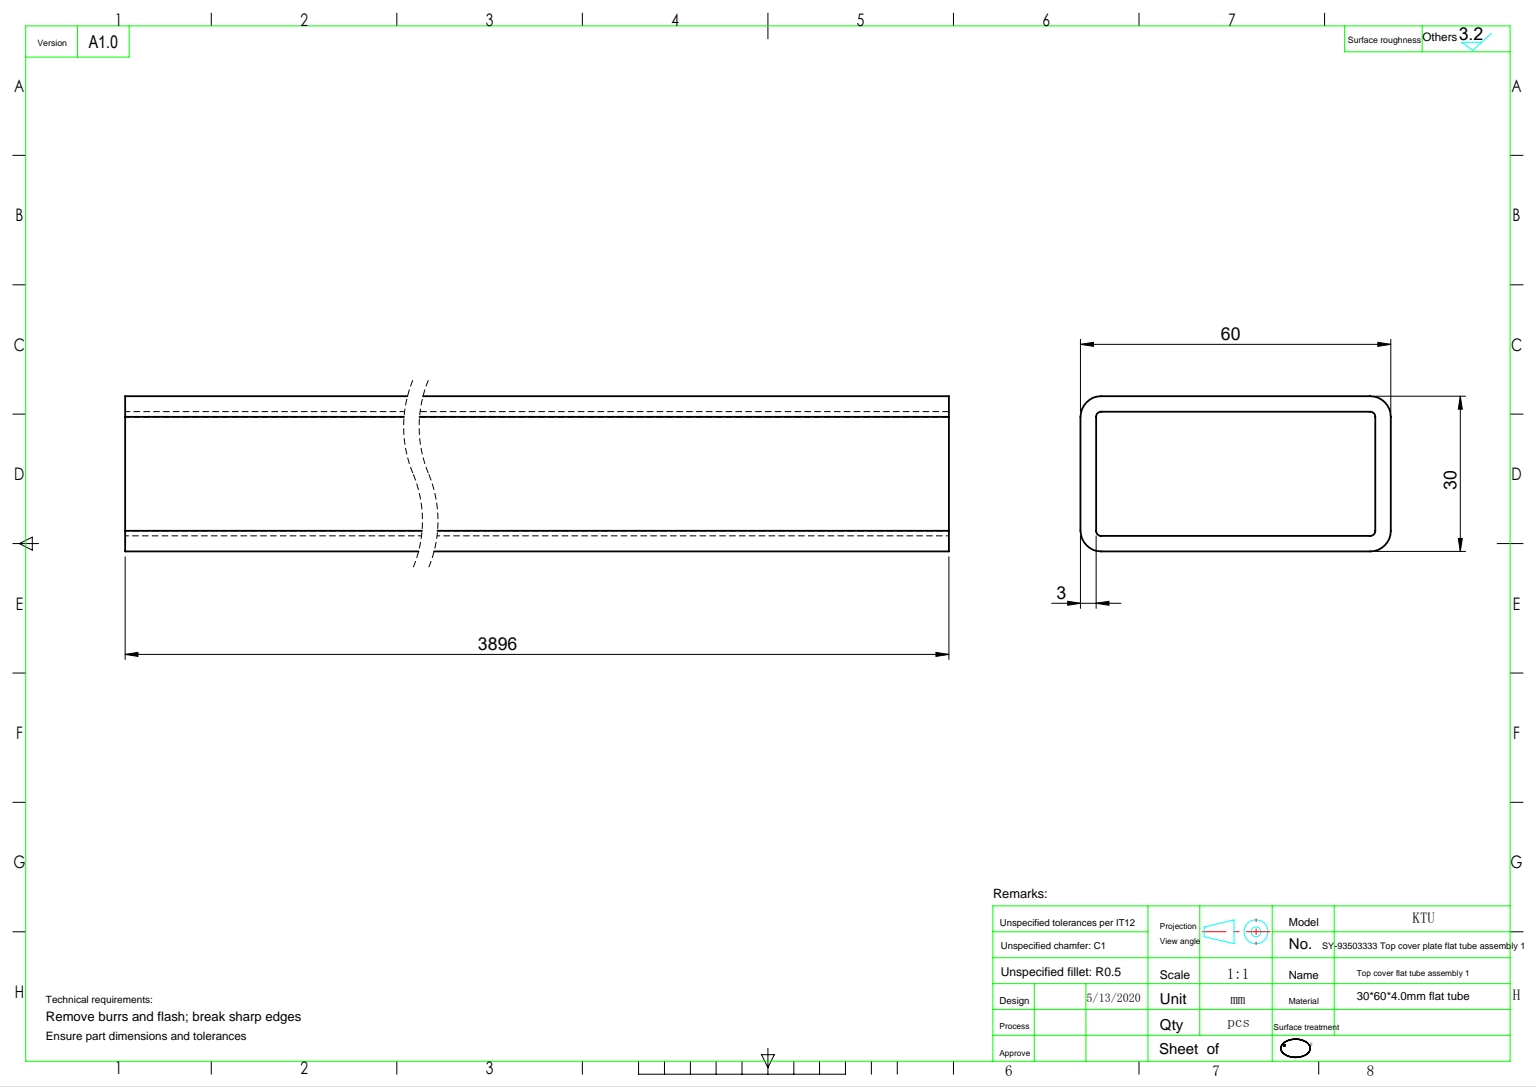
SolidWorks part; units mm, degrees
ref_plane "前视基准面" through (0, 0, 0) normal (0, 0, 1) x (1, 0, 0)
ref_plane "上视基准面" through (0, 0, 0) normal (0, 1, 0) x (1, 0, 0)
ref_plane "右视基准面" through (0, 0, 0) normal (1, 0, 0) x (0, 0, -1)
sketch "草图1" plane through (0, 0, 0) normal (0, 0, 1) x (1, 0, 0)
  line L1 (-26, 15) -> (26, 15)
  line L2 (-30, 11) -> (-30, -11)
  line L3 (-26, -15) -> (26, -15)
  line L4 (30, 11) -> (30, -11)
  line L5 (-30, 15) -> (30, -15) construction
  line L6 (-30, -15) -> (30, 15) construction
  arc A0 (26, 15) -> (30, 11) centre (26, 11) cw
  arc A1 (26, -15) -> (30, -11) centre (26, -11) ccw
  arc A2 (-30, -11) -> (-26, -15) centre (-26, -11) ccw
  arc A3 (-26, 15) -> (-30, 11) centre (-26, 11) ccw
  point P0 (0, 0)
  dimension "D3" = 4
  dimension "D1" = 60
  dimension "D2" = 30
extrude "拉伸-薄壁1" add sketch "草图1" along normal mid plane 3896 thin
